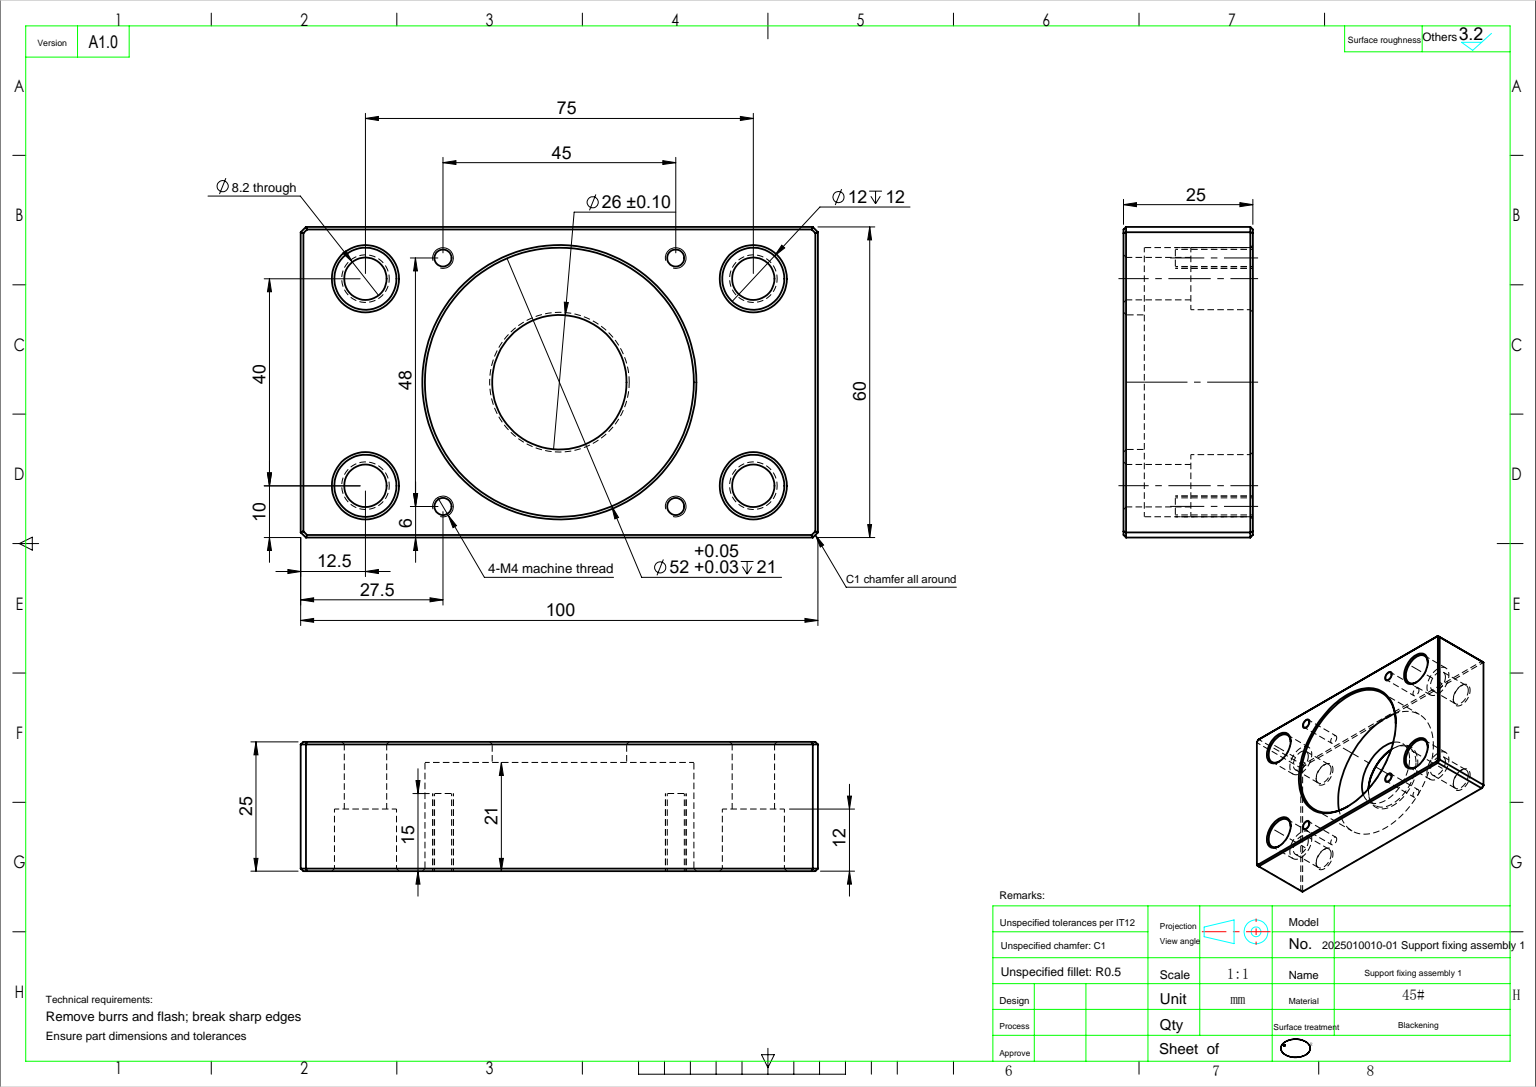
from build123d import *

# Parameters (mm, degrees)
SKETCH_1_W          = 100
SKETCH_1_H          = 60
EXTRUDE_1_DEPTH     = 25
SKETCH_2_R          = 13
CUT_EXTRUDE_1_DEPTH = 64.442887702
SKETCH_3_R          = 6
CUT_EXTRUDE_2_DEPTH = 12
SKETCH_4_R          = 4.1
CUT_EXTRUDE_3_DEPTH = 64.442887702
CHAMFER_1_SIZE      = 1
CHAMFER_4_SIZE      = 0.5
SKETCH_8_R          = 26
CUT_EXTRUDE_5_DEPTH = 21
CHAMFER_5_SIZE      = 0.5
SKETCH_9_R          = 1.65
CUT_EXTRUDE_6_DEPTH = 15


with BuildPart() as part:
    # 草图1 → 凸台-拉伸1 (new body)
    with BuildSketch(Plane.XY):
        Rectangle(SKETCH_1_W, SKETCH_1_H)
    extrude(amount=EXTRUDE_1_DEPTH)

    # 草图2 → 切除-拉伸1 (cut, through all)
    with BuildSketch(Plane.XY.offset(25)):
        Circle(SKETCH_2_R)
    extrude(amount=-CUT_EXTRUDE_1_DEPTH, mode=Mode.SUBTRACT)

    # 草图3 → 切除-拉伸2 (cut)
    with BuildSketch(Plane.XY.offset(25)):
        with Locations((-37.5, 20)):
            Circle(SKETCH_3_R)
        with Locations((-37.5, -20)):
            Circle(SKETCH_3_R)
        with Locations((37.5, -20)):
            Circle(SKETCH_3_R)
        with Locations((37.5, 20)):
            Circle(SKETCH_3_R)
    extrude(amount=-CUT_EXTRUDE_2_DEPTH, mode=Mode.SUBTRACT)

    # 草图4 → 切除-拉伸3 (cut, through all)
    with BuildSketch(Plane.XY.offset(25)):
        with Locations((-37.5, 20)):
            Circle(SKETCH_4_R)
        with Locations((-37.5, -20)):
            Circle(SKETCH_4_R)
        with Locations((37.5, 20)):
            Circle(SKETCH_4_R)
        with Locations((37.5, -20)):
            Circle(SKETCH_4_R)
    extrude(amount=-CUT_EXTRUDE_3_DEPTH, mode=Mode.SUBTRACT)

    # 倒角1
    chamfer_1_edges = [part.edges().sort_by_distance(p)[0] for p in [
        (50, -30, 12.5),
        (-50, -30, 12.5),
        (-50, 30, 12.5),
        (50, 30, 12.5),
    ]]
    chamfer(chamfer_1_edges, length=CHAMFER_1_SIZE)

    # 倒角4
    chamfer_4_edges = [part.edges().sort_by_distance(p)[0] for p in [
        (-13, 0, 0),
        (-41.6, -20, 0),
        (33.4, 20, 0),
        (33.4, -20, 0),
        (-41.6, 20, 0),
        (-50, 0, 0),
        (50, 0, 0),
        (0, -30, 0),
        (0, 30, 0),
        (-49.5, -29.5, 0),
        (49.5, -29.5, 0),
        (49.5, 29.5, 0),
        (-49.5, 29.5, 0),
    ]]
    chamfer(chamfer_4_edges, length=CHAMFER_4_SIZE)

    # 草图8 → 切除-拉伸5 (cut)
    with BuildSketch(Plane.XY.offset(25)):
        Circle(SKETCH_8_R)
    extrude(amount=-CUT_EXTRUDE_5_DEPTH, mode=Mode.SUBTRACT)

    # 倒角5
    chamfer_5_edges = [part.edges().sort_by_distance(p)[0] for p in [
        (-26, 0, 25),
        (31.5, 20, 25),
        (31.5, -20, 25),
        (-43.5, -20, 25),
        (-43.5, 20, 25),
        (-50, 0, 25),
        (0, 30, 25),
        (50, 0, 25),
        (0, -30, 25),
        (-49.5, -29.5, 25),
        (49.5, -29.5, 25),
        (49.5, 29.5, 25),
        (-49.5, 29.5, 25),
    ]]
    chamfer(chamfer_5_edges, length=CHAMFER_5_SIZE)

    # 草图9 → 切除-拉伸6 (cut)
    with BuildSketch(Plane.XY.offset(25)):
        with Locations((22.5, -24)):
            Circle(SKETCH_9_R)
        with Locations((22.5, 24)):
            Circle(SKETCH_9_R)
        with Locations((-22.5, 24)):
            Circle(SKETCH_9_R)
        with Locations((-22.5, -24)):
            Circle(SKETCH_9_R)
    extrude(amount=-CUT_EXTRUDE_6_DEPTH, mode=Mode.SUBTRACT)


solid = part.part
